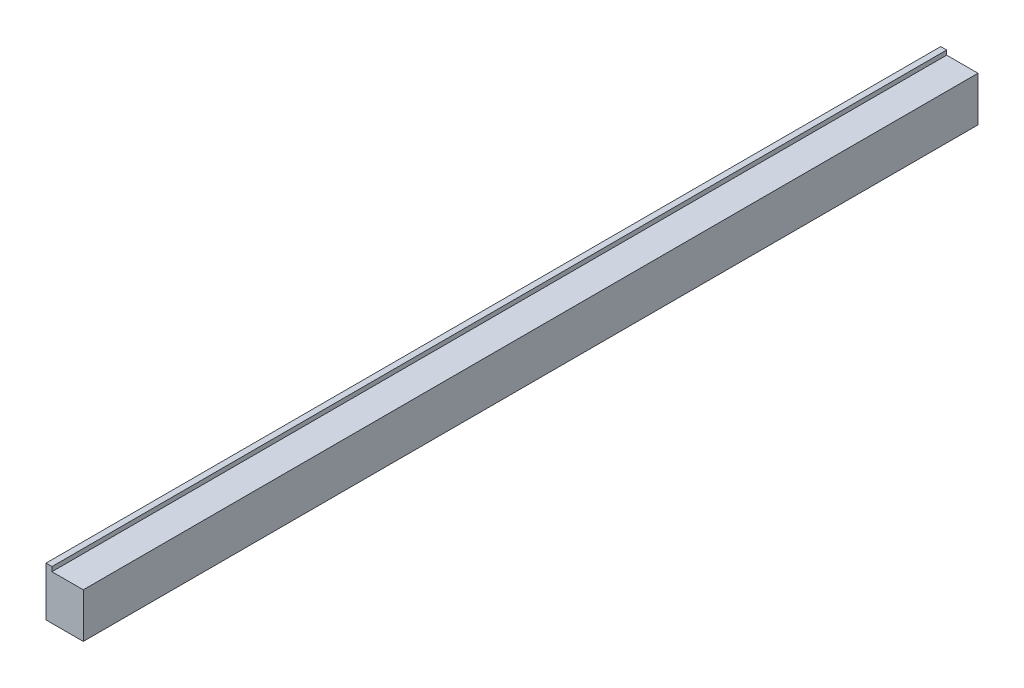
SolidWorks part; units mm, degrees
ref_plane "前视基准面" through (0, 0, 0) normal (0, 0, 1) x (1, 0, 0)
ref_plane "上视基准面" through (0, 0, 0) normal (0, 1, 0) x (1, 0, 0)
ref_plane "右视基准面" through (0, 0, 0) normal (1, 0, 0) x (0, 0, -1)
sketch "草图1" plane through (0, 0, -300) normal (0, 0, 1) x (1, 0, 0)
  line L0 (-10, -12.5) -> (-14, -12.5)
  line L1 (-10, -10.2831) -> (-10, -14.5) construction
  line L2 (-14, -12.5) -> (-14, -45.5)
  line L3 (-14, -45.5) -> (11, -45.5)
  line L4 (11, -45.5) -> (11, -15.5)
  line L5 (11, -15.5) -> (-10, -15.5)
  line L6 (-10, -15.5) -> (-10, -12.5)
  dimension "D1" = 30
  dimension "D2" = 3
  dimension "D3" = 4
  dimension "D4" = 25
  dimension "D5" = 15.5
extrude "凸台-拉伸1" add sketch "草图1" against normal up to surface (600 mm away)
